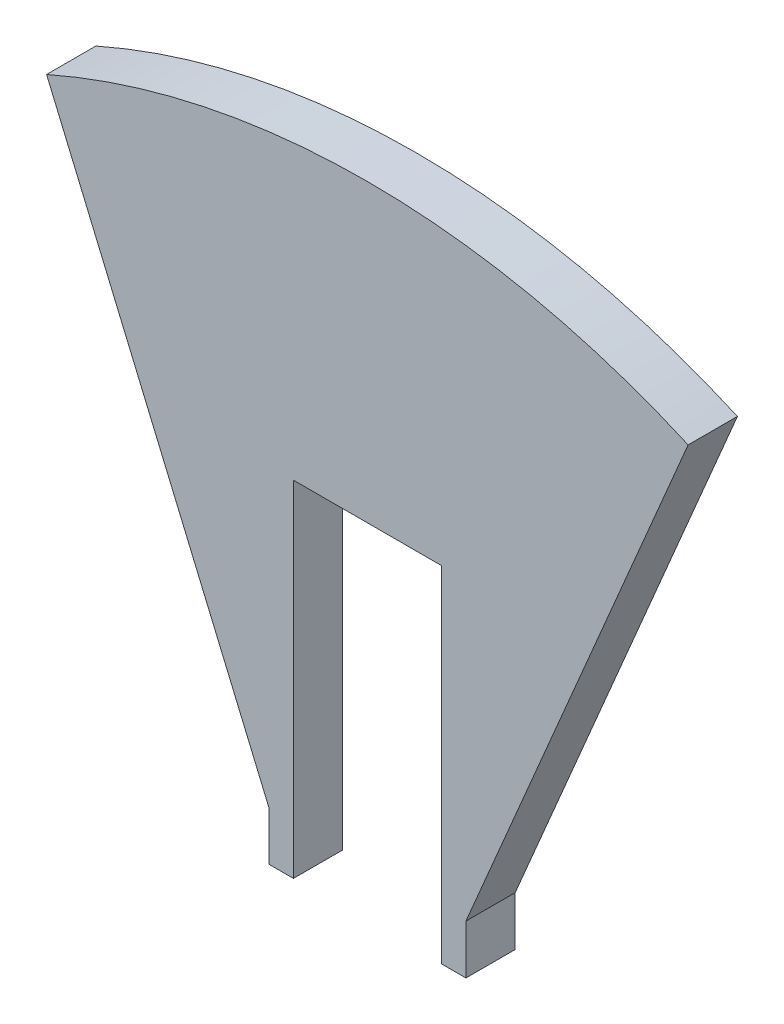
from build123d import *

# Parameters (mm, degrees)
BOSS_EXTRUDE2_DEPTH = 5


with BuildPart() as part:
    # Sketch1 → Boss-Extrude2 (new, symmetric)
    with BuildSketch(Plane.XY):
        with BuildLine():
            ThreePointArc((65.10089705, 147.251055016), (0, 161), (-65.10089705, 147.251055016))
            Line((-65.10089705, 147.251055016), (-20, 41))
            Line((-20, 41), (-20, 31))
            Line((-20, 31), (-15, 31))
            Line((-15, 31), (-15, 101))
            Line((-15, 101), (15, 101))
            Line((15, 101), (15, 31))
            Line((15, 31), (20, 31))
            Line((20, 31), (20, 41))
            Line((20, 41), (65.10089705, 147.251055016))
        make_face()
    extrude(amount=BOSS_EXTRUDE2_DEPTH, both=True)


solid = part.part
